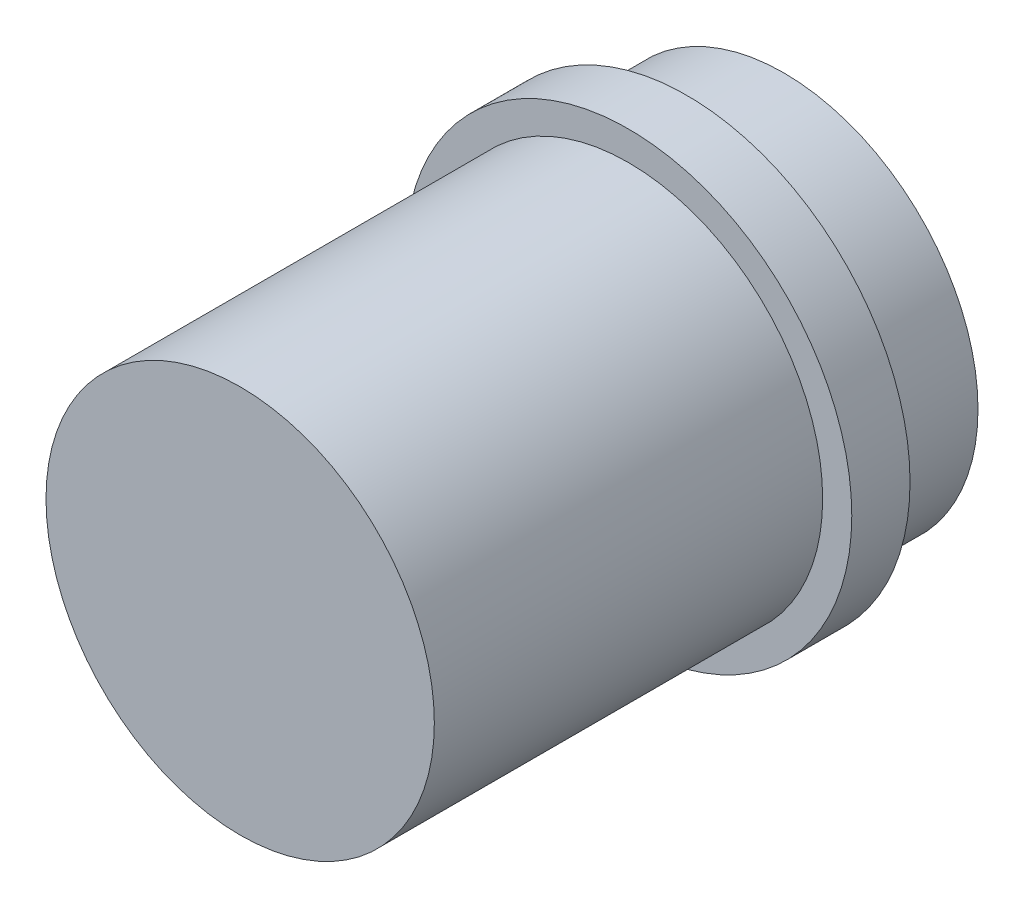
SolidWorks part; units mm, degrees
ref_plane "Front Plane" through (0, 0, 0) normal (0, 0, 1) x (1, 0, 0)
ref_plane "Top Plane" through (0, 0, 0) normal (0, 1, 0) x (1, 0, 0)
ref_plane "Right Plane" through (0, 0, 0) normal (1, 0, 0) x (0, 0, -1)
other "Configuration Table"
sketch "Sketch1" plane through (0, 0, 0) normal (0, 0, 1) x (1, 0, 0)
  circle A0 centre (0, 0) radius 10
  dimension "D1" = 20
extrude "Boss-Extrude2" add sketch "Sketch1" along normal blind 5
sketch "Sketch2" plane through (0, 0, 5) normal (0, 0, 1) x (1, 0, 0)
  circle A0 centre (0, 0) radius 11.5
  dimension "D1" = 23
extrude "Boss-Extrude3" add sketch "Sketch2" along normal blind 3
sketch "Sketch3" plane through (0, 0, 8) normal (0, 0, 1) x (1, 0, 0)
  circle A0 centre (0, 0) radius 10
  dimension "D1" = 20
extrude "Boss-Extrude4" add sketch "Sketch3" along normal blind 20
